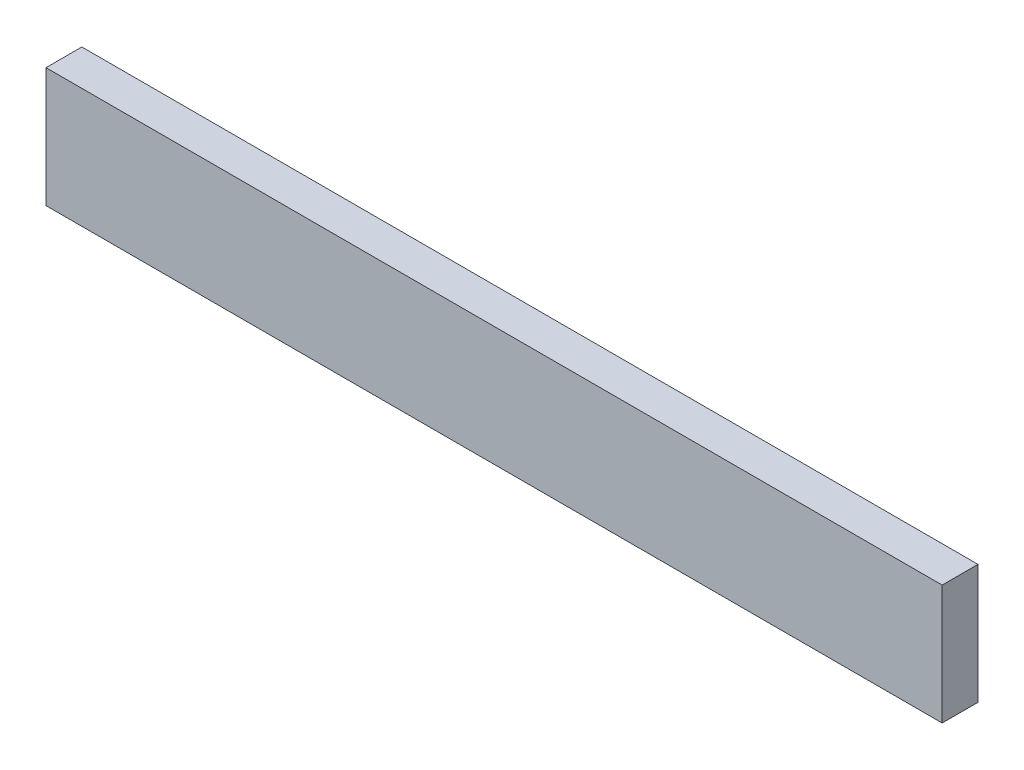
SolidWorks part; units mm, degrees
ref_plane "前视基准面" through (0, 0, 0) normal (0, 0, 1) x (1, 0, 0)
ref_plane "上视基准面" through (0, 0, 0) normal (0, 1, 0) x (1, 0, 0)
ref_plane "右视基准面" through (0, 0, 0) normal (1, 0, 0) x (0, 0, -1)
sketch "草图1" plane through (0, 0, 0) normal (0, 0, 1) x (1, 0, 0)
  line L1 (-75, -10) -> (75, -10)
  line L2 (-75, -10) -> (-75, 10)
  line L3 (-75, 10) -> (75, 10)
  line L4 (75, -10) -> (75, 10)
  line L5 (-75, -10) -> (75, 10) construction
  line L6 (-75, 10) -> (75, -10) construction
  point P0 (0, 0)
  dimension "D1" = 20
  dimension "D2" = 150
extrude "凸台-拉伸1" add sketch "草图1" along normal blind 6
